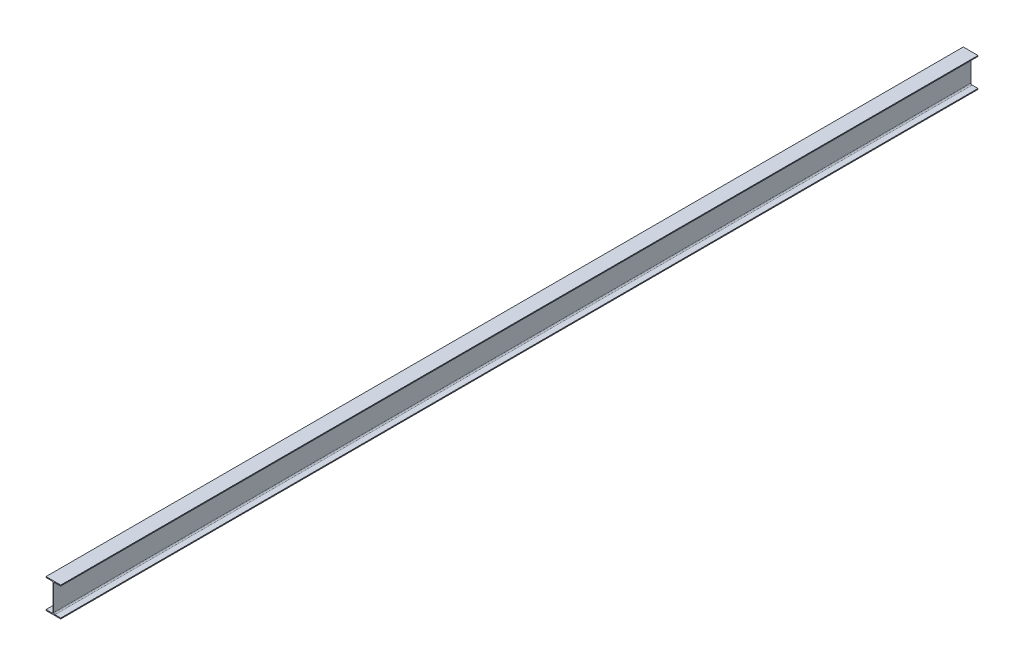
from build123d import *

# Parameters (mm, degrees)
BOSS_EXTRUDE1_DEPTH = 9347


with BuildPart() as part:
    # Sketch1 → Boss-Extrude1 (new body)
    with BuildSketch(Plane.XY):
        with BuildLine():
            Line((75, 0), (-75, 0))
            Line((-75, 0), (-75, 9))
            Line((-75, 9), (-16.25, 9))
            ThreePointArc((-16.25, 9), (-7.057611845, 12.807611845), (-3.25, 22))
            Line((-3.25, 22), (-3.25, 278))
            ThreePointArc((-3.25, 278), (-7.057611845, 287.192388155), (-16.25, 291))
            Line((-16.25, 291), (-75, 291))
            Line((-75, 291), (-75, 300))
            Line((-75, 300), (75, 300))
            Line((75, 300), (75, 291))
            Line((75, 291), (16.25, 291))
            ThreePointArc((16.25, 291), (7.057611845, 287.192388155), (3.25, 278))
            Line((3.25, 278), (3.25, 22))
            ThreePointArc((3.25, 22), (7.057611845, 12.807611845), (16.25, 9))
            Line((16.25, 9), (75, 9))
            Line((75, 9), (75, 0))
        make_face()
    extrude(amount=BOSS_EXTRUDE1_DEPTH)


solid = part.part
